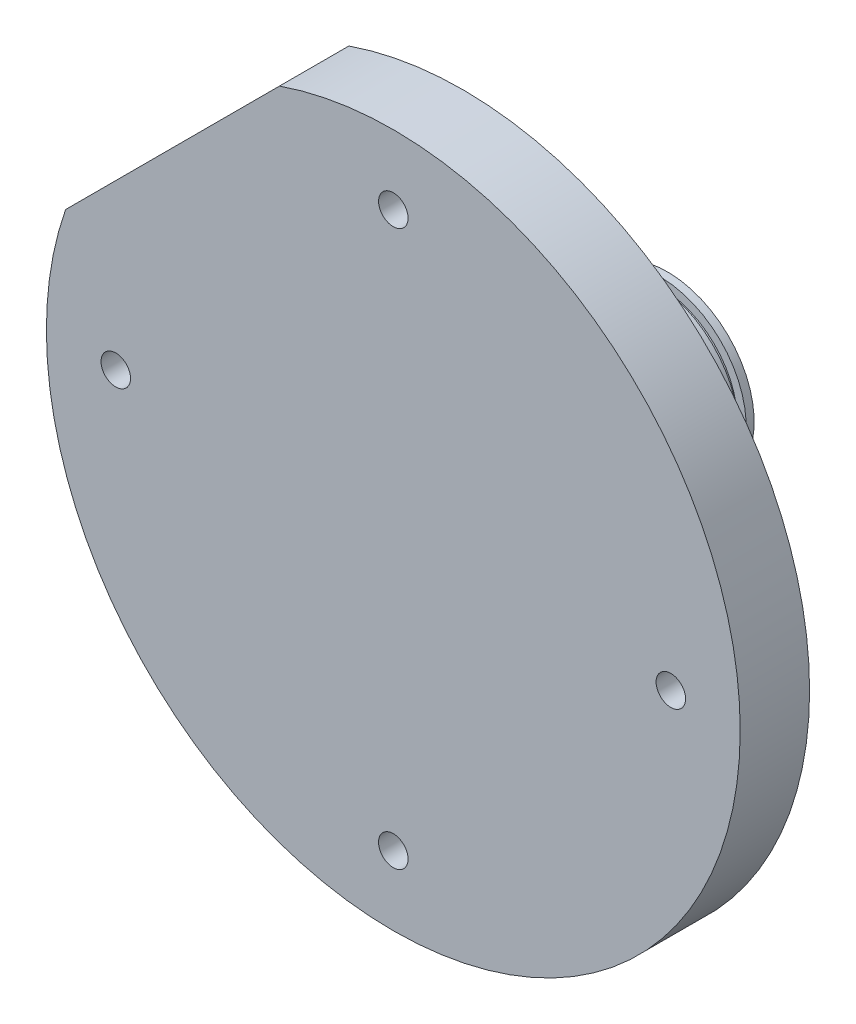
SolidWorks part; units mm, degrees
ref_plane "前视基准面" through (0, 0, 0) normal (0, 0, 1) x (1, 0, 0)
ref_plane "上视基准面" through (0, 0, 0) normal (0, 1, 0) x (1, 0, 0)
ref_plane "右视基准面" through (0, 0, 0) normal (1, 0, 0) x (0, 0, -1)
sketch "草图1" plane through (0, 0, 0) normal (0, 1, 0) x (1, 0, 0)
  line L0 (0, 0) -> (0, -33070.6301) construction
  line L1 (0, 0) -> (-100, 0)
  line L2 (-100, 0) -> (-100, 20)
  line L3 (-100, 20) -> (-26.5, 20)
  line L4 (-26.5, 20) -> (-26.5, 49.02)
  line L5 (-26.5, 49.02) -> (-25, 49.02)
  line L6 (-25, 49.02) -> (-25, 79.02)
  line L7 (-25, 79.02) -> (0, 79.02)
  line L8 (0, 79.02) -> (0, 0)
  dimension "D1" = 49.02
  dimension "D2" = 30
  dimension "D3" = 53
  dimension "D4" = 50
  dimension "D5" = 20
  dimension "D6" = 100
revolve "旋转1" add sketch "草图1" angle 360 about L0
ref_plane "基准面1" through (0, 0, -74.52) normal (0, 0, -1) x (-1, 0, 0)
sketch "草图4" plane through (0, 0, -74.52) normal (0, 0, -1) x (-1, 0, 0)
  circle A0 centre (0, 0) radius 22.5
  circle A4 centre (0, 0) radius 25 construction
  dimension "D1" = 2.5
extrude "切除-拉伸2" cut sketch "草图4" along normal blind 2.2 flip side to cut
hole_wizard "M10 螺纹孔1" positions "草图8" profile "草图9" tap size "M10" standard "GB" end condition through all
sketch "草图8" plane through (0, 0, -20) normal (0, 0, -1) x (-1, 0, 0)
  point P0 (0, -80)
  dimension "D1" = 80
sketch "草图9" plane through (0, -80, -20) normal (1, 0, 0) x (0, 1, 0)
  line L0 (0, 0) -> (0, 20)
  line L1 (0, 20) -> (4.25, 20)
  line L2 (4.25, 20) -> (4.25, 0)
  line L5 (4.25, 0) -> (0, 0)
  line L11 (0, -6.35) -> (0, 107.95) construction
  dimension "通孔螺纹孔钻头直径" = 8.5
  dimension "通孔螺纹孔钻头深度" = 20
cosmetic thread "孔螺蚊线5" parameters "D2"=10
pattern_circular "阵列(圆周)1" count 4 over 360 about axis through (0, 0, 0) along (0, 0, 1) of "M10 螺纹孔1"
sketch "草图10" plane through (0, 0, -20) normal (0, 0, -1) x (-1, 0, 0)
  line L0 (-80, 0) -> (0, -80) construction
  line L1 (0, -80) -> (80, 0) construction
  line L2 (80, 0) -> (0, 80) construction
  line L3 (0, 80) -> (-80, 0) construction
  line L4 (106.066, 21.2132) -> (21.2132, 106.066)
  line L5 (21.2132, 106.066) -> (56.7861, 141.6389)
  line L6 (56.7861, 141.6389) -> (141.6389, 56.7861)
  line L7 (141.6389, 56.7861) -> (106.066, 21.2132)
  circle A1 centre (0, 0) radius 100 construction
  dimension "D1" = 10
  dimension "D2" = 60
  dimension "D3" = 60
extrude "切除-拉伸5" cut sketch "草图10" against normal through all
hole_wizard "M10 螺纹孔2" positions "草图11" profile "草图12" tap size "M10" standard "GB"
sketch "草图11" plane through (-63.6396, 63.6396, 0) normal (-0.7071, 0.7071, 0) x (0.7071, 0.7071, 0)
  point P0 (0, 12)
  dimension "D1" = 12
sketch "草图12" plane through (-63.6396, 63.6396, -12) normal (0, 0, 1) x (-0.7071, -0.7071, 0)
  line L0 (0, 0) -> (0, 62.5537)
  line L1 (0, 62.5537) -> (4.25, 60)
  line L2 (4.25, 60) -> (4.25, 0)
  line L5 (4.25, 0) -> (0, 0)
  line L10 (0, 62.5537) -> (-4.25, 60) construction
  line L11 (0, -6.35) -> (0, 107.95) construction
  dimension "螺纹孔钻头直径" = 8.5
  dimension "螺纹孔钻头深度" = 60
  dimension "导头角度" = 118
cosmetic thread "孔螺蚊线6" parameters "D1"=55, "D2"=10
